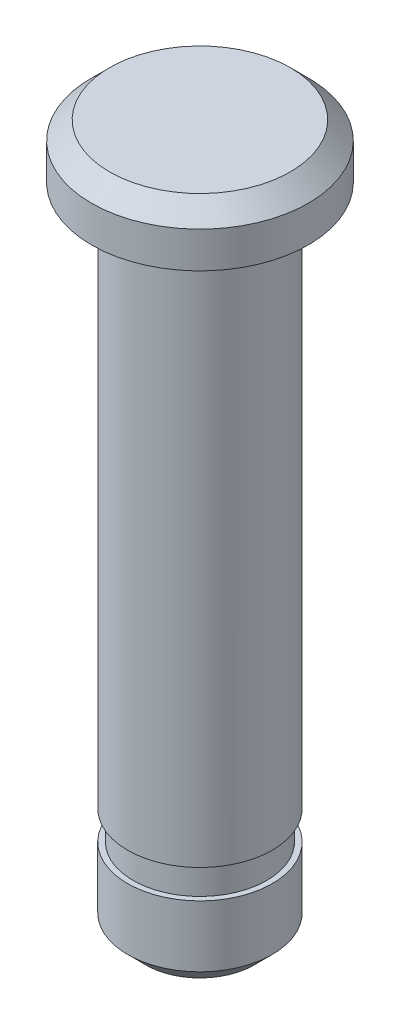
SolidWorks part; units mm, degrees
material "SUS304"
ref_plane "Front Plane" through (0, 0, 0) normal (0, 0, 1) x (1, 0, 0)
ref_plane "Top Plane" through (0, 0, 0) normal (0, 1, 0) x (1, 0, 0)
ref_plane "Right Plane" through (0, 0, 0) normal (1, 0, 0) x (0, 0, -1)
sketch "Sketch1" plane through (0, 0, 0) normal (0, 1, 0) x (1, 0, 0)
  circle A0 centre (0, 0) radius 3
  dimension "D1" = 6
extrude "Boss-Extrude1" add sketch "Sketch1" along normal blind 1.5
sketch "Sketch2" plane through (0, 0, 0) normal (0, -1, 0) x (1, 0, 0)
  circle A0 centre (0, 0) radius 2
  dimension "D1" = 4
extrude "Boss-Extrude2" add sketch "Sketch2" along normal blind 18
sketch "Sketch3" plane through (0, 0, 0) normal (1, 0, 0) x (0, 0, -1)
  line L0 (2, -18) -> (2, 0) construction
  line L1 (2, -15) -> (1.85, -15)
  line L2 (2, -15) -> (2, -15.8)
  line L3 (2, -15.8) -> (1.85, -15.8)
  line L4 (1.85, -15) -> (1.85, -15.8)
  line L5 (3, 1.5) -> (-3, 1.5) construction
  line L6 (0, -16.5635) -> (0, 1.3658) construction
  dimension "D1" = 16.5
  dimension "D2" = 0.8
  dimension "D3" = 0.15
revolve "Cut-Revolve1" cut sketch "Sketch3" angle 360 about L6
chamfer "Chamfer1" distance 0.5 angle 45 2 edges at (0, -18, -2) (0, 1.5, 3)
chamfer "Chamfer2" [suppressed] distance 0.25 angle 45
